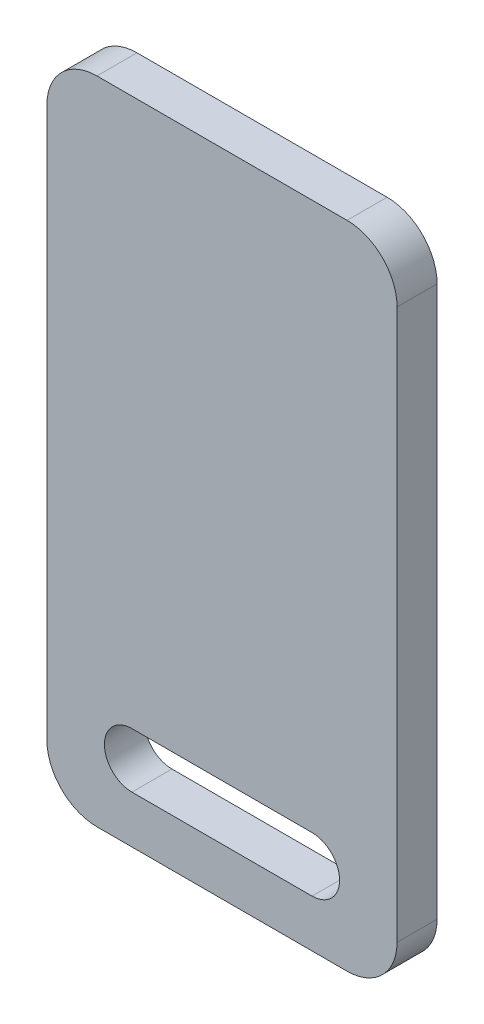
from build123d import *

# Parameters (mm, degrees)
BOSS_EXTRUDE1_DEPTH = 8
CUT_EXTRUDE1_DEPTH  = 10


with BuildPart() as part:
    # Sketch1 → Boss-Extrude1 (new body)
    with BuildSketch(Plane.XY):
        with BuildLine():
            Line((10, 0), (60, 0))
            ThreePointArc((60, 0), (67.071067812, 2.928932188), (70, 10))
            Line((70, 10), (70, 120))
            ThreePointArc((70, 120), (67.071067812, 127.071067812), (60, 130))
            Line((60, 130), (10, 130))
            ThreePointArc((10, 130), (2.928932188, 127.071067812), (0, 120))
            Line((0, 120), (0, 10))
            ThreePointArc((0, 10), (2.928932188, 2.928932188), (10, 0))
        make_face()
    extrude(amount=BOSS_EXTRUDE1_DEPTH)

    # Sketch2 → Cut-Extrude1 (cut)
    with BuildSketch(Plane.XY.offset(8)):
        with BuildLine():
            Line((17, 20.5), (53, 20.5))
            ThreePointArc((53, 20.5), (58.5, 15), (53, 9.5))
            Line((53, 9.5), (17, 9.5))
            ThreePointArc((17, 9.5), (11.5, 15), (17, 20.5))
        make_face()
    extrude(amount=-CUT_EXTRUDE1_DEPTH, mode=Mode.SUBTRACT)


solid = part.part
